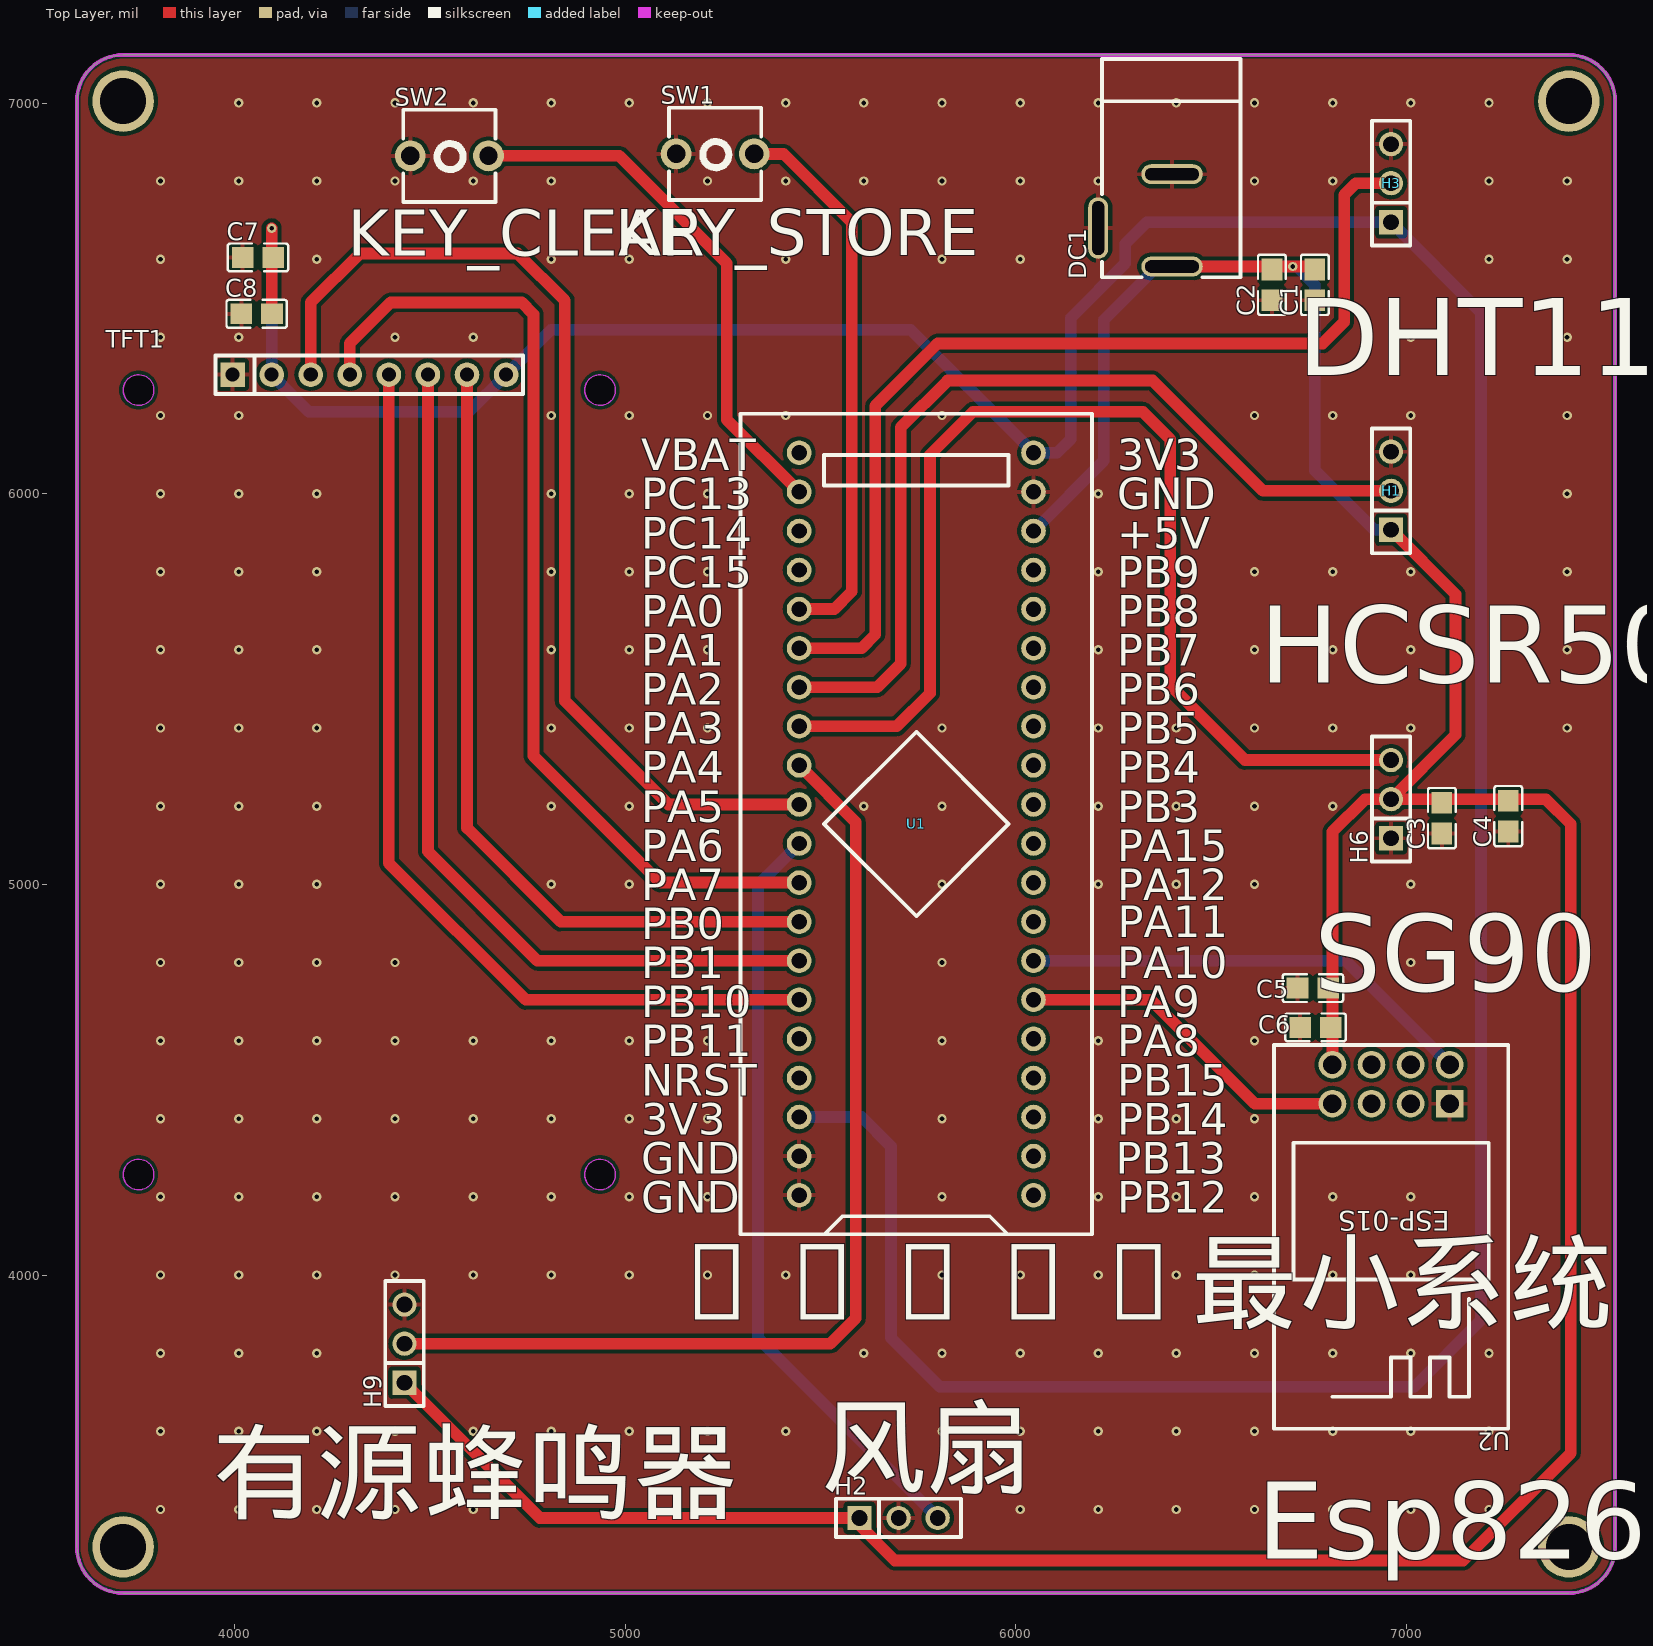
[diagram p0: Top Layer view]
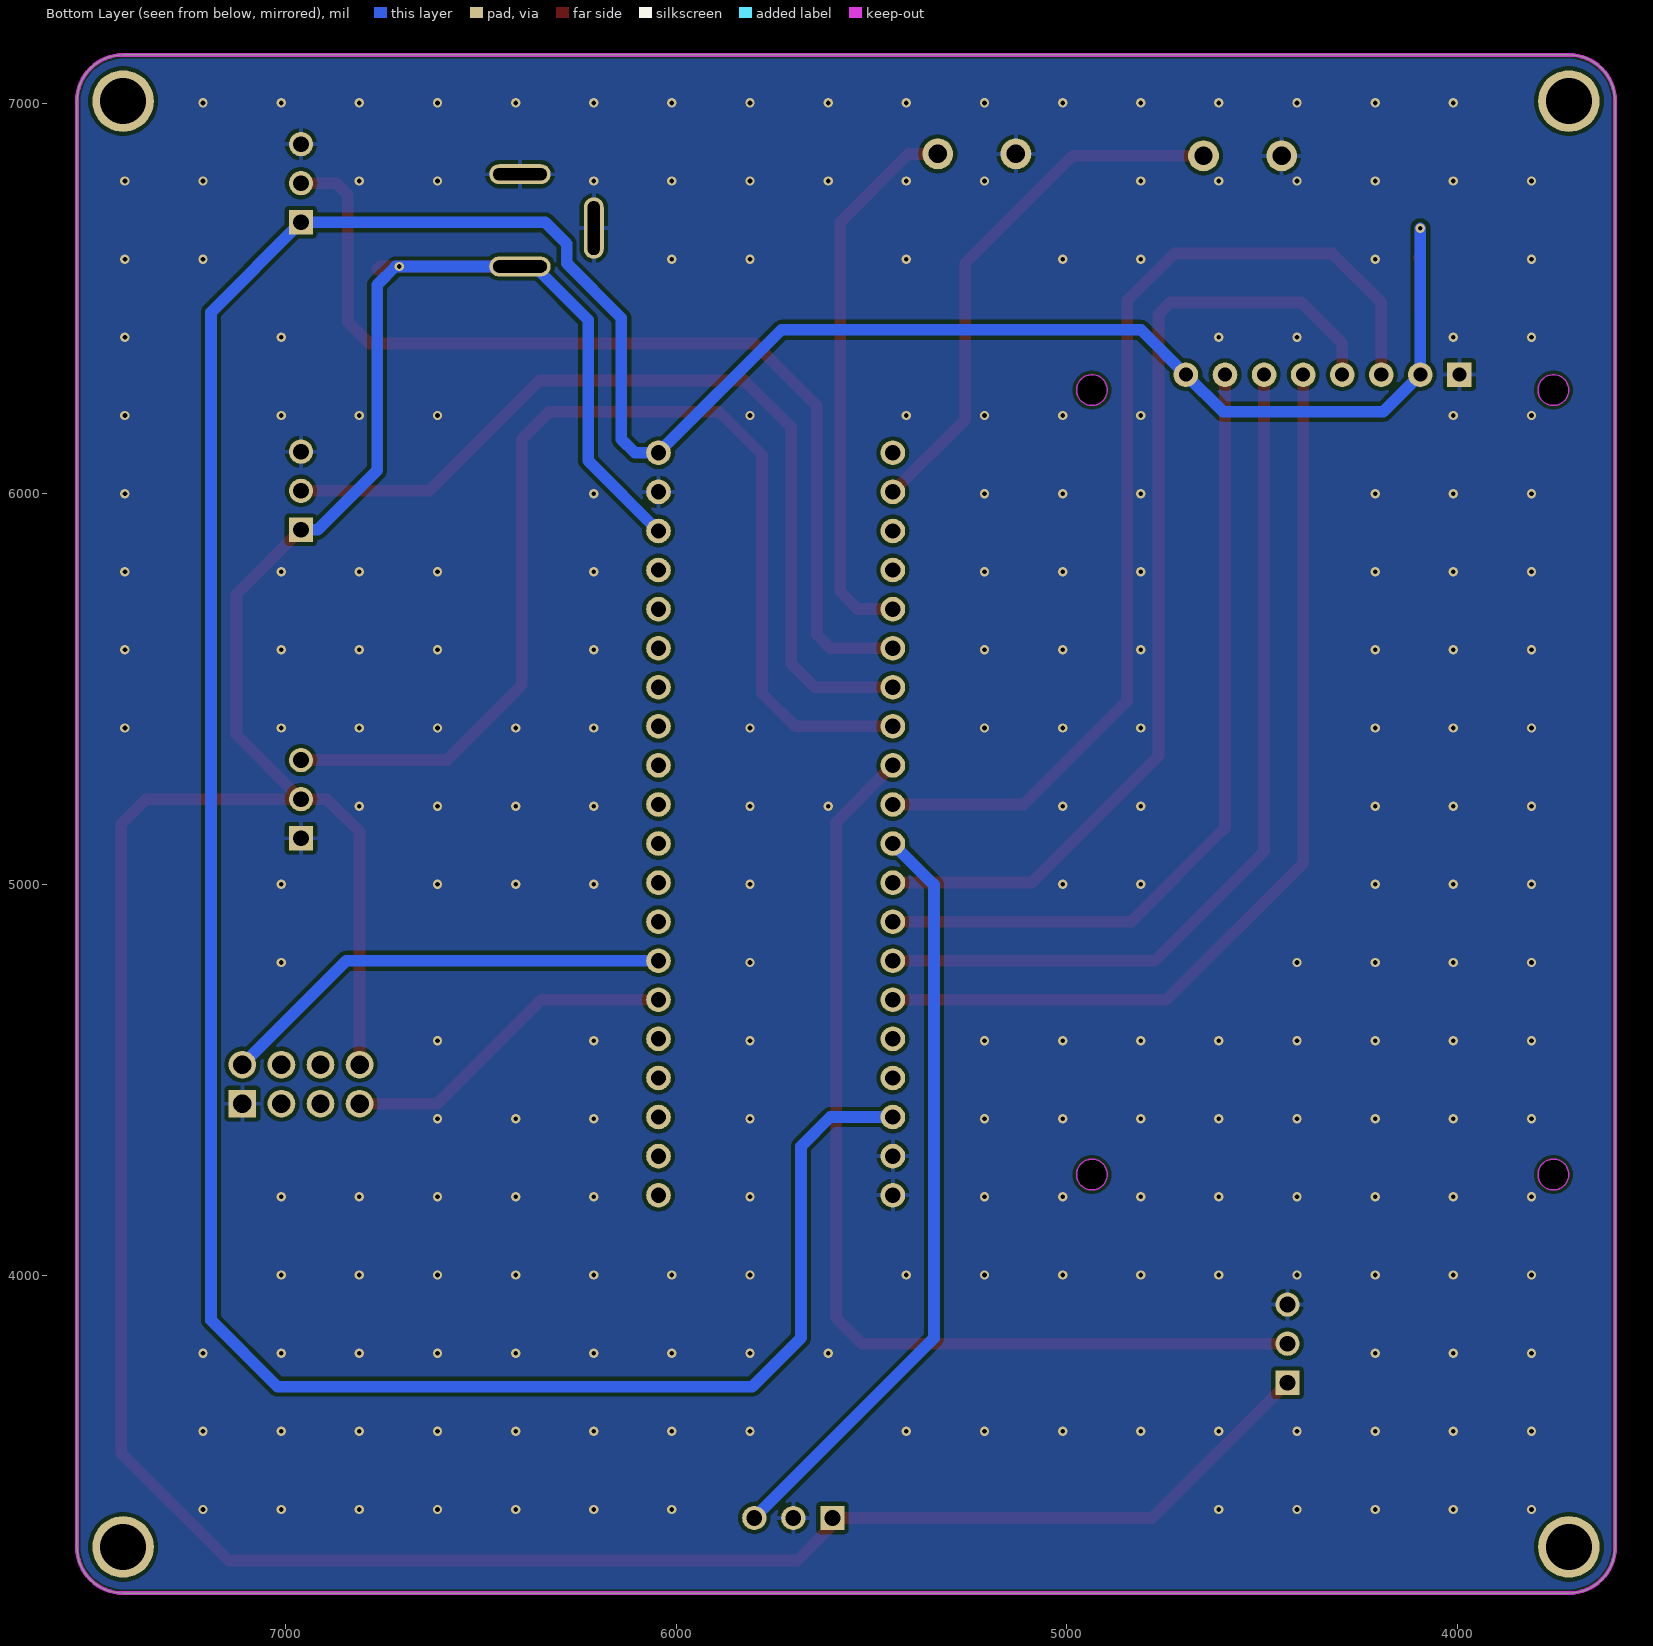
[diagram p1: Bottom Layer view, seen from below]
# Altium PCB MISC52046.pcbdoc
Units mil, origin at the board's own origin, x right, y up, seen from the top; angles counter-clockwise.
Board outline 3937.01 x 3937.01 mil, 2 copper layers (Top Layer, Bottom Layer), stack 62.206 mil thick; 19 components, 37 nets, 98 pads, 225 vias.

## Layer stack, top to bottom
Top Solder Mask Layer: solder mask 0.394, Dk 3.3
Top Layer: signal copper 1.379
Dielectric1: surface 59.449, FR4, Dk 4.5
Bottom Layer: signal copper 1.378
Bottom Solder Mask Layer: solder mask 0.394, Dk 3.3

## Board outline
3714.61,7123.5 ccw(c3714.61,7005.39) 3596.5,7005.39 3596.5,3304.61 ccw(c3714.61,3304.61) 3714.61,3186.5 7415.39,3186.5 ccw(c7415.39,3304.61) 7533.5,3304.61 7533.5,7005.39 ccw(c7415.39,7005.39) 7415.39,7123.5 3714.61,7123.5

## Design rules (kind name [scope] priority, off if disabled: settings)
BoardOutlineClearance copperThickness2oz_1 [All] p2 off: genericclearance=7.99 ignorepadtopadclearanceinfootprint=FALSE except(0: Arc-SplitContinuation Track-SplitContinuation SMDPad-SplitContinuation THPad-SplitContinuation Via-SplitContinuation Fill-SplitContinuation Region-SplitContinuation Poly-SplitContinuation Text-SplitContinuation Hole-SplitContinuation; 5.98: Arc-CutoutEdge Track-CutoutEdge SMDPad-CutoutEdge THPad-CutoutEdge Via-CutoutEdge Text-CutoutEdge; 6.9: Hole-OutlineEdge Hole-CutoutEdge; 10: Poly-OutlineEdge Poly-CutoutEdge; 11.81: Arc-OutlineEdge Track-OutlineEdge SMDPad-OutlineEdge THPad-OutlineEdge Via-OutlineEdge Fill-OutlineEdge Region-OutlineEdge Text-OutlineEdge Fill-CutoutEdge Region-CutoutEdge)
BoardOutlineClearance Plane_innerPlane_1 [All] p4 off: genericclearance=4.02 ignorepadtopadclearanceinfootprint=FALSE except(0: Arc-SplitContinuation Track-SplitContinuation SMDPad-SplitContinuation THPad-SplitContinuation Via-SplitContinuation Fill-SplitContinuation Region-SplitContinuation Poly-SplitContinuation Text-SplitContinuation Hole-SplitContinuation; 5.98: Arc-CutoutEdge Track-CutoutEdge SMDPad-CutoutEdge THPad-CutoutEdge Via-CutoutEdge Text-CutoutEdge; 6.9: Hole-OutlineEdge Hole-CutoutEdge; 10: Poly-OutlineEdge Poly-CutoutEdge; 11.81: Arc-OutlineEdge Track-OutlineEdge SMDPad-OutlineEdge THPad-OutlineEdge Via-OutlineEdge Fill-OutlineEdge Region-OutlineEdge Text-OutlineEdge Fill-CutoutEdge Region-CutoutEdge)
BoardOutlineClearance Copper_copperRegion_1 [All] p6 off: genericclearance=4.02 ignorepadtopadclearanceinfootprint=FALSE except(0: Arc-SplitContinuation Track-SplitContinuation SMDPad-SplitContinuation THPad-SplitContinuation Via-SplitContinuation Fill-SplitContinuation Region-SplitContinuation Poly-SplitContinuation Text-SplitContinuation Hole-SplitContinuation; 5.98: Arc-CutoutEdge Track-CutoutEdge SMDPad-CutoutEdge THPad-CutoutEdge Via-CutoutEdge Text-CutoutEdge; 6.9: Hole-OutlineEdge Hole-CutoutEdge; 10: Poly-OutlineEdge Poly-CutoutEdge; 11.81: Arc-OutlineEdge Track-OutlineEdge SMDPad-OutlineEdge THPad-OutlineEdge Via-OutlineEdge Fill-OutlineEdge Region-OutlineEdge Text-OutlineEdge Fill-CutoutEdge Region-CutoutEdge)
BoardOutlineClearance Copper_copperRegion_copperThickness1oz_1 [All] p8 off: genericclearance=4.02 ignorepadtopadclearanceinfootprint=FALSE except(0: Arc-SplitContinuation Track-SplitContinuation SMDPad-SplitContinuation THPad-SplitContinuation Via-SplitContinuation Fill-SplitContinuation Region-SplitContinuation Poly-SplitContinuation Text-SplitContinuation Hole-SplitContinuation; 5.98: Arc-CutoutEdge Track-CutoutEdge SMDPad-CutoutEdge THPad-CutoutEdge Via-CutoutEdge Text-CutoutEdge; 6.9: Hole-OutlineEdge Hole-CutoutEdge; 10: Poly-OutlineEdge Poly-CutoutEdge; 11.81: Arc-OutlineEdge Track-OutlineEdge SMDPad-OutlineEdge THPad-OutlineEdge Via-OutlineEdge Fill-OutlineEdge Region-OutlineEdge Text-OutlineEdge Fill-CutoutEdge Region-CutoutEdge)
BoardOutlineClearance Copper_copperRegion_Copper_copperRegion_1 [All] p10 off: genericclearance=4.02 ignorepadtopadclearanceinfootprint=FALSE except(0: Arc-SplitContinuation Track-SplitContinuation SMDPad-SplitContinuation THPad-SplitContinuation Via-SplitContinuation Fill-SplitContinuation Region-SplitContinuation Poly-SplitContinuation Text-SplitContinuation Hole-SplitContinuation; 5.98: Arc-CutoutEdge Track-CutoutEdge SMDPad-CutoutEdge THPad-CutoutEdge Via-CutoutEdge Text-CutoutEdge; 6.9: Hole-OutlineEdge Hole-CutoutEdge; 10: Poly-OutlineEdge Poly-CutoutEdge; 11.81: Arc-OutlineEdge Track-OutlineEdge SMDPad-OutlineEdge THPad-OutlineEdge Via-OutlineEdge Fill-OutlineEdge Region-OutlineEdge Text-OutlineEdge Fill-CutoutEdge Region-CutoutEdge)
BoardOutlineClearance copperThickness1oz_1 [All] p12: genericclearance=4.02 ignorepadtopadclearanceinfootprint=FALSE except(0: Arc-SplitContinuation Track-SplitContinuation SMDPad-SplitContinuation THPad-SplitContinuation Via-SplitContinuation Fill-SplitContinuation Region-SplitContinuation Poly-SplitContinuation Text-SplitContinuation Hole-SplitContinuation; 5.98: Arc-CutoutEdge Track-CutoutEdge SMDPad-CutoutEdge THPad-CutoutEdge Via-CutoutEdge Text-CutoutEdge; 6.9: Hole-OutlineEdge Hole-CutoutEdge; 10: Poly-OutlineEdge Poly-CutoutEdge; 11.81: Arc-OutlineEdge Track-OutlineEdge SMDPad-OutlineEdge THPad-OutlineEdge Via-OutlineEdge Fill-OutlineEdge Region-OutlineEdge Text-OutlineEdge Fill-CutoutEdge Region-CutoutEdge)
Clearance copperThickness2oz [All] p1 off: gap=7.99 ignorepadtopadclearanceinfootprint=FALSE except(5.98: SMDPad-Track SMDPad-SMDPad THPad-Track SMDPad-THPad THPad-THPad Track-Via SMDPad-Via THPad-Via Via-Via Fill-SMDPad Region-SMDPad Fill-THPad Region-THPad Fill-Via Region-Via Fill-Fill Fill-Region Region-Region Arc-Track Arc-SMDPad Arc-THPad Arc-Via Fill-Arc Region-Arc Arc-Arc Text-Track SMDPad-Text Text-THPad Text-Via Fill-Text Region-Text Arc-Text Text-Text; 6.9: Hole-Track Hole-SMDPad Hole-THPad Hole-Via Fill-Hole Region-Hole Hole-Arc Hole-Text; 10: Poly-Track Poly-SMDPad Poly-THPad Poly-Via Poly-Fill Poly-Region Poly-Poly Poly-Arc Poly-Text Poly-Hole; 11.81: Fill-Track Region-Track)
Clearance Plane_innerPlane [All] p3 off: gap=4.02 ignorepadtopadclearanceinfootprint=FALSE except(5.98: SMDPad-Track SMDPad-SMDPad THPad-Track SMDPad-THPad THPad-THPad Track-Via SMDPad-Via THPad-Via Via-Via Fill-SMDPad Region-SMDPad Fill-THPad Region-THPad Fill-Via Region-Via Fill-Fill Fill-Region Region-Region Arc-Track Arc-SMDPad Arc-THPad Arc-Via Fill-Arc Region-Arc Arc-Arc Text-Track SMDPad-Text Text-THPad Text-Via Fill-Text Region-Text Arc-Text Text-Text; 6.9: Hole-Track Hole-SMDPad Hole-THPad Hole-Via Fill-Hole Region-Hole Hole-Arc Hole-Text; 10: Poly-Track Poly-SMDPad Poly-THPad Poly-Via Poly-Fill Poly-Region Poly-Poly Poly-Arc Poly-Text Poly-Hole; 11.81: Fill-Track Region-Track)
Clearance Copper_copperRegion [All] p5 off: gap=4.02 ignorepadtopadclearanceinfootprint=FALSE except(5.98: SMDPad-Track SMDPad-SMDPad THPad-Track SMDPad-THPad THPad-THPad Track-Via SMDPad-Via THPad-Via Via-Via Fill-SMDPad Region-SMDPad Fill-THPad Region-THPad Fill-Via Region-Via Fill-Fill Fill-Region Region-Region Arc-Track Arc-SMDPad Arc-THPad Arc-Via Fill-Arc Region-Arc Arc-Arc Text-Track SMDPad-Text Text-THPad Text-Via Fill-Text Region-Text Arc-Text Text-Text; 6.9: Hole-Track Hole-SMDPad Hole-THPad Hole-Via Fill-Hole Region-Hole Hole-Arc Hole-Text; 10: Poly-Track Poly-SMDPad Poly-THPad Poly-Via Poly-Fill Poly-Region Poly-Poly Poly-Arc Poly-Text Poly-Hole; 11.81: Fill-Track Region-Track)
Clearance Copper_copperRegion_copperThickness1oz [All] p7 off: gap=4.02 ignorepadtopadclearanceinfootprint=FALSE except(5.98: SMDPad-Track SMDPad-SMDPad THPad-Track SMDPad-THPad THPad-THPad Track-Via SMDPad-Via THPad-Via Via-Via Fill-SMDPad Region-SMDPad Fill-THPad Region-THPad Fill-Via Region-Via Fill-Fill Fill-Region Region-Region Arc-Track Arc-SMDPad Arc-THPad Arc-Via Fill-Arc Region-Arc Arc-Arc Text-Track SMDPad-Text Text-THPad Text-Via Fill-Text Region-Text Arc-Text Text-Text; 6.9: Hole-Track Hole-SMDPad Hole-THPad Hole-Via Fill-Hole Region-Hole Hole-Arc Hole-Text; 10: Poly-Track Poly-SMDPad Poly-THPad Poly-Via Poly-Fill Poly-Region Poly-Poly Poly-Arc Poly-Text Poly-Hole; 11.81: Fill-Track Region-Track)
Clearance Copper_copperRegion_Copper_copperRegion [All] p9 off: gap=4.02 ignorepadtopadclearanceinfootprint=FALSE except(5.98: SMDPad-Track SMDPad-SMDPad THPad-Track SMDPad-THPad THPad-THPad Track-Via SMDPad-Via THPad-Via Via-Via Fill-SMDPad Region-SMDPad Fill-THPad Region-THPad Fill-Via Region-Via Fill-Fill Fill-Region Region-Region Arc-Track Arc-SMDPad Arc-THPad Arc-Via Fill-Arc Region-Arc Arc-Arc Text-Track SMDPad-Text Text-THPad Text-Via Fill-Text Region-Text Arc-Text Text-Text; 6.9: Hole-Track Hole-SMDPad Hole-THPad Hole-Via Fill-Hole Region-Hole Hole-Arc Hole-Text; 10: Poly-Track Poly-SMDPad Poly-THPad Poly-Via Poly-Fill Poly-Region Poly-Poly Poly-Arc Poly-Text Poly-Hole; 11.81: Fill-Track Region-Track)
Clearance copperThickness1oz [All] p11: gap=4.02 ignorepadtopadclearanceinfootprint=FALSE except(5.98: SMDPad-Track SMDPad-SMDPad THPad-Track SMDPad-THPad THPad-THPad Track-Via SMDPad-Via THPad-Via Via-Via Fill-SMDPad Region-SMDPad Fill-THPad Region-THPad Fill-Via Region-Via Fill-Fill Fill-Region Region-Region Arc-Track Arc-SMDPad Arc-THPad Arc-Via Fill-Arc Region-Arc Arc-Arc Text-Track SMDPad-Text Text-THPad Text-Via Fill-Text Region-Text Arc-Text Text-Text; 6.9: Hole-Track Hole-SMDPad Hole-THPad Hole-Via Fill-Hole Region-Hole Hole-Arc Hole-Text; 10: Poly-Track Poly-SMDPad Poly-THPad Poly-Via Poly-Fill Poly-Region Poly-Poly Poly-Arc Poly-Text Poly-Hole; 11.81: Fill-Track Region-Track)
DiffPairsRouting differentialPair [All] p1: maxlimit=6 minlimit=6 mostfreqgap=6 toplayer_minwidth=5 toplayer_prefwidth=10 toplayer_maxwidth=100 toplayer_mingap=6 toplayer_prefgap=6 toplayer_maxgap=6 bottomlayer_minwidth=5 bottomlayer_prefwidth=10 bottomlayer_maxwidth=100 bottomlayer_mingap=6 bottomlayer_prefgap=6 bottomlayer_maxgap=6 maxuncoupledlength=10
HoleToHoleClearance otherClearance [All] p1: gap=11.81 allowstackedmicrovias=TRUE
Length netLength [All] p1: minlimit=0 maxlimit=0
PasteMaskExpansion pasteMaskExpansion [All] p1: expansion=0
PlaneConnect innerPlane [All] p1: planeconnectstyle=Relief reliefexpansion=20 reliefentries=4 reliefconductorwidth=10 reliefairgap=10
PolygonConnect copperRegion_copperThickness1oz [All] p1 off: connectstyle=Relief reliefconductorwidth=10 reliefentries=4 polygonreliefangle="90 Angle" airgapwidth=10 via.connectstyle=Relief via.reliefconductorwidth=10 via.reliefentries=4 via.polygonreliefangle="90 Angle" via.airgapwidth=10
PolygonConnect copperRegion_Copper_copperRegion [All] p2 off: connectstyle=Relief reliefconductorwidth=10 reliefentries=4 polygonreliefangle="90 Angle" airgapwidth=10 via.connectstyle=Relief via.reliefconductorwidth=10 via.reliefentries=4 via.polygonreliefangle="90 Angle" via.airgapwidth=10
PolygonConnect copperRegion [All] p3: connectstyle=Relief reliefconductorwidth=10 reliefentries=4 polygonreliefangle="90 Angle" airgapwidth=10 via.connectstyle=Relief via.reliefconductorwidth=10 via.reliefentries=4 via.polygonreliefangle="90 Angle" via.airgapwidth=10
RoutingVias viaSize [All] p1: holewidth=12.01 width=24.02 viastyle="Through Hole" minholewidth=11.81 minwidth=19.68 maxholewidth=248.03 maxwidth=393.7
SolderMaskExpansion solderMaskExpansion [IsVia] p1: expansion=-1000 istentingtop=TRUE
SolderMaskExpansion solderMaskExpansion [All] p2: expansion=2 istentingtop=FALSE
Width copperThickness2oz_2 [All] p1 off: maxlimit=100 minlimit=8 preferedwidth=10
Width copperThickness1oz_2 [All] p2: maxlimit=100 minlimit=5 preferedwidth=10

## Components (designator, comment, footprint, x,y, rotation, side; value= is the part's Value field where it differs from the comment)
C1 "100uF" C0805 6765,6535 r90 top
C2 "100nF" C0805 6655,6535 r90 top
C3 "470uF" C0805 7090,5170 r90 top
C4 "100nF" C0805 7260,5175 r90 top
C5 "100uF" C0805 6760,4735 r0 top
C6 "100nF" C0805 6766.7,4634.47 r0 top
C7 "10uF" C0805 4060,6605 r0 top
C8 "100nF" C0805 4056.7,6460.8 r0 top
DC1 "" DC-2.0 6410,6705 r90 top
H1 "" HDR-TH_3P-P2.54-V-F 6960,6007.85 r90 top
H2 "" HDR-TH_3P-P2.54-V-F 5699.74,3378.84 r0 top
H3 "" HDR-TH_3P-P2.54-V-F 6960,6795 r90 top
H6 "" HDR-TH_3P-P2.54-V-F 6960,5218.61 r90 top
H9 "" HDR-TH_3P-P2.54-V-F 4435,3825 r90 top
SW1 "OMRON_B3F-6000" KEY-TH_2P-L6.0-W6.0-P5.00 5230,6870 r0 top
SW2 "OMRON_B3F-6000" KEY-TH_2P-L6.0-W6.0-P5.00 4550,6865 r0 top
TFT1 "1.8 TFT 128*RGB*160" LCD-TH_8P-P2.54-L56.0-W34.0_1.8-TFT 4345,6305 r0 top
U1 "STM32F103C8T6-Card" CONN-TH_L53.3-W22.9_STM32F103C8T6-CARD 5745,5155 r90 top
U2 "ESP-01S" WIFIM-TH_ESP-01S 6960,4489.11 r180 top

## Footprints (in the part's own frame and the unit in brackets; to place one, negate y for a bottom-side part, rotate by r counter-clockwise, add the part's x,y. Pads: shape width x height; smd on the part's side, far side on the other; paste and mask are expansions set on the pad)
C0805 [mm]
  rect 1.41x1.35 smd paste-100 mask+0.051: 1(-1,0) 2(1,0)
  silkscreen extent -1.96,-0.9 1.96,0.9
CONN-TH_L53.3-W22.9_STM32F103C8T6-CARD [mm]
  round 1.6 hole 1: 1(-24.13,-7.62) 2(-21.59,-7.62) 3(-19.05,-7.62) 4(-16.51,-7.62) 5(-13.97,-7.62) 6(-11.43,-7.62) 7(-8.89,-7.62) 8(-6.35,-7.62) 9(-3.81,-7.62) 10(-1.27,-7.62) 11(1.27,-7.62) 12(3.81,-7.62) 13(6.35,-7.62) 14(8.89,-7.62) 15(11.43,-7.62) 16(13.97,-7.62) 17(16.51,-7.62) 18(19.05,-7.62) 19(21.59,-7.62) 20(24.13,-7.62) 21(24.13,7.62) 22(21.59,7.62) 23(19.05,7.62) 24(16.51,7.62) 25(13.97,7.62) 26(11.43,7.62) 27(8.89,7.62) 28(6.35,7.62) 29(3.81,7.62) 30(1.27,7.62) 31(-1.27,7.62) 32(-3.81,7.62) 33(-6.35,7.62) 34(-8.89,7.62) 35(-11.43,7.62) 36(-13.97,7.62) 37(-16.51,7.62) 38(-19.05,7.62) 39(-21.59,7.62) 40(-24.13,7.62)
  silkscreen extent -26.67,-11.43 26.67,11.43
DC-2.0 [mil]
  oval 157.5x51.2 hole 31.5 slot 137.8 at 0 deg paste+0 mask+2: 2(-24.7,199.5)
  oval 51.2x157.5 hole 31.5 slot 137.8 at 90 deg paste+0 mask+2: 3(113.1,10.5) 4(-123.1,10.5)
  silkscreen extent -151,-165 408,190
HDR-TH_3P-P2.54-V-F [mil]
  rect 62x62 hole 40.16: 1(-100,0)
  round 62 hole 40.16: 2(0,0) 3(100,0)
  silkscreen extent -160,-49 160,49
KEY-TH_2P-L6.0-W6.0-P5.00 [mm]
  round 2 hole 1.2: 1(-2.54,0) 2(2.54,0)
  silkscreen extent -3,-3 3,3
LCD-TH_8P-P2.54-L56.0-W34.0_1.8-TFT [mm]
  rect 1.6x1.6 hole 0.914: 1(-8.89,0)
  round 1.6 hole 0.914: 2(-6.35,0) 3(-3.81,0) 4(-1.27,0) 5(1.27,0) 6(3.81,0) 7(6.35,0) 8(8.89,0)
  Board Outline Layer circle w0.003: c15,-1 r1
  Board Outline Layer circle w0.003: c-15,-1 r1
  Board Outline Layer circle w0.003: c15,-52 r1
  Board Outline Layer circle w0.003: c-15,-52 r1
  Board Outline Layer region: 16,-1 15.901,-1.434 15.623,-1.782 15.222,-1.975 14.777,-1.975 14.376,-1.782 14.099,-1.434 14,-1 14,-1 14.099,-0.566 14.376,-0.218 14.777,-0.025 15.222,-0.025 15.623,-0.218 15.901,-0.566 16,-1
  Board Outline Layer region: 16,-1 15.991,-1.136 15.963,-1.27 15.917,-1.398 15.854,-1.52 15.776,-1.631 15.683,-1.731 15.577,-1.817 15.46,-1.888 15.335,-1.942 15.203,-1.979 15.068,-1.998 14.932,-1.998 14.797,-1.979 14.665,-1.942 14.54,-1.888 14.423,-1.817 14.317,-1.731 14.224,-1.631 14.146,-1.52 14.083,-1.398 14.037,-1.27 14.009,-1.136 14,-1 14.009,-0.864 14.037,-0.73 14.083,-0.602 14.146,-0.48 14.224,-0.369 14.317,-0.269 14.423,-0.183 14.54,-0.112 14.665,-0.058 14.797,-0.021 14.932,-0.002 15.068,-0.002 15.203,-0.021 15.335,-0.058 15.46,-0.112 15.577,-0.183 15.683,-0.269 15.776,-0.369 15.854,-0.48 15.917,-0.602 15.963,-0.73 15.991,-0.864
  Board Outline Layer region: -14,-1 -14.099,-1.434 -14.376,-1.782 -14.777,-1.975 -15.222,-1.975 -15.623,-1.782 -15.901,-1.434 -16,-1 -16,-1 -15.901,-0.566 -15.623,-0.218 -15.222,-0.025 -14.777,-0.025 -14.376,-0.218 -14.099,-0.566 -14,-1
  Board Outline Layer region: -14,-1 -14.009,-1.136 -14.037,-1.27 -14.083,-1.398 -14.146,-1.52 -14.224,-1.631 -14.317,-1.731 -14.423,-1.817 -14.54,-1.888 -14.665,-1.942 -14.797,-1.979 -14.932,-1.998 -15.068,-1.998 -15.203,-1.979 -15.335,-1.942 -15.46,-1.888 -15.577,-1.817 -15.683,-1.731 -15.776,-1.631 -15.854,-1.52 -15.917,-1.398 -15.963,-1.27 -15.991,-1.136 -16,-1 -15.991,-0.864 -15.963,-0.73 -15.917,-0.602 -15.854,-0.48 -15.776,-0.369 -15.683,-0.269 -15.577,-0.183 -15.46,-0.112 -15.335,-0.058 -15.203,-0.021 -15.068,-0.002 -14.932,-0.002 -14.797,-0.021 -14.665,-0.058 -14.54,-0.112 -14.423,-0.183 -14.317,-0.269 -14.224,-0.369 -14.146,-0.48 -14.083,-0.602 -14.037,-0.73 -14.009,-0.864
  Board Outline Layer region: 16,-52 15.901,-52.434 15.623,-52.782 15.222,-52.975 14.777,-52.975 14.376,-52.782 14.099,-52.434 14,-52 14,-52 14.099,-51.566 14.376,-51.218 14.777,-51.025 15.222,-51.025 15.623,-51.218 15.901,-51.566 16,-52
  Board Outline Layer region: 16,-52 15.991,-52.136 15.963,-52.27 15.917,-52.398 15.854,-52.519 15.776,-52.631 15.683,-52.731 15.577,-52.817 15.46,-52.888 15.335,-52.942 15.203,-52.979 15.068,-52.998 14.932,-52.998 14.797,-52.979 14.665,-52.942 14.54,-52.888 14.423,-52.817 14.317,-52.731 14.224,-52.631 14.146,-52.519 14.083,-52.398 14.037,-52.27 14.009,-52.136 14,-52 14.009,-51.864 14.037,-51.73 14.083,-51.601 14.146,-51.48 14.224,-51.369 14.317,-51.269 14.423,-51.183 14.54,-51.112 14.665,-51.058 14.797,-51.021 14.932,-51.002 15.068,-51.002 15.203,-51.021 15.335,-51.058 15.46,-51.112 15.577,-51.183 15.683,-51.269 15.776,-51.369 15.854,-51.48 15.917,-51.601 15.963,-51.73 15.991,-51.864
  Board Outline Layer region: -14,-52 -14.099,-52.434 -14.376,-52.782 -14.777,-52.975 -15.222,-52.975 -15.623,-52.782 -15.901,-52.434 -16,-52 -16,-52 -15.901,-51.566 -15.623,-51.218 -15.222,-51.025 -14.777,-51.025 -14.376,-51.218 -14.099,-51.566 -14,-52
  Board Outline Layer region: -14,-52 -14.009,-52.136 -14.037,-52.27 -14.083,-52.398 -14.146,-52.519 -14.224,-52.631 -14.317,-52.731 -14.423,-52.817 -14.54,-52.888 -14.665,-52.942 -14.797,-52.979 -14.932,-52.998 -15.068,-52.998 -15.203,-52.979 -15.335,-52.942 -15.46,-52.888 -15.577,-52.817 -15.683,-52.731 -15.776,-52.631 -15.854,-52.519 -15.917,-52.398 -15.963,-52.27 -15.991,-52.136 -16,-52 -15.991,-51.864 -15.963,-51.73 -15.917,-51.601 -15.854,-51.48 -15.776,-51.369 -15.683,-51.269 -15.577,-51.183 -15.46,-51.112 -15.335,-51.058 -15.203,-51.021 -15.068,-51.002 -14.932,-51.002 -14.797,-51.021 -14.665,-51.058 -14.54,-51.112 -14.423,-51.183 -14.317,-51.269 -14.224,-51.369 -14.146,-51.48 -14.083,-51.601 -14.037,-51.73 -14.009,-51.864
  Multi-Layer board cut-out: 16,-1 15.901,-1.434 15.623,-1.782 15.222,-1.975 14.777,-1.975 14.376,-1.782 14.099,-1.434 14,-1 14,-1 14.099,-0.566 14.376,-0.218 14.777,-0.025 15.222,-0.025 15.623,-0.218 15.901,-0.566 16,-1
  Multi-Layer board cut-out: -14,-1 -14.099,-1.434 -14.376,-1.782 -14.777,-1.975 -15.222,-1.975 -15.623,-1.782 -15.901,-1.434 -16,-1 -16,-1 -15.901,-0.566 -15.623,-0.218 -15.222,-0.025 -14.777,-0.025 -14.376,-0.218 -14.099,-0.566 -14,-1
  Multi-Layer board cut-out: 16,-52 15.901,-52.434 15.623,-52.782 15.222,-52.975 14.777,-52.975 14.376,-52.782 14.099,-52.434 14,-52 14,-52 14.099,-51.566 14.376,-51.218 14.777,-51.025 15.222,-51.025 15.623,-51.218 15.901,-51.566 16,-52
  Multi-Layer board cut-out: -14,-52 -14.099,-52.434 -14.376,-52.782 -14.777,-52.975 -15.222,-52.975 -15.623,-52.782 -15.901,-52.434 -16,-52 -16,-52 -15.901,-51.566 -15.623,-51.218 -15.222,-51.025 -14.777,-51.025 -14.376,-51.218 -14.099,-51.566 -14,-52
  silkscreen extent -10,-1.25 10,1.25
WIFIM-TH_ESP-01S [mm]
  rect 1.8x1.8 hole 1.2: 1(-3.81,1.27)
  round 1.8 hole 1.2: 2(-1.27,1.27) 3(1.27,1.27) 4(3.81,1.27) 5(3.81,-1.27) 6(1.27,-1.27) 7(-1.27,-1.27) 8(-3.81,-1.27)
  silkscreen extent -7.62,-2.54 7.62,22.4

## Free pads (board coordinates)
  round 157.48 hole 118.11: 1(3714.61,7005.39) 1(3714.61,3304.61) 1(7415.39,7005.39) 1(7415.39,3304.61)

## Via types
v1: diameter 24.02, hole 12, Top Layer to Bottom Layer, 225 vias

## Nets (pads, with @x,y where several pads share a name; then routed paths per layer and width w, separated by ;. In a path a pad name is that pad's centre, name@x,y a point inside that pad or via, vN(x,y) a via of type N, cw(c..) or ccw(c..) an arc to the next point about the centre after c; other vN are vias at no path point)
+5V: C1.2 C2.2 C3.2 C4.2 C5.2 C6.2 DC1.4 H1.1 H2.1 H6.2 H9.1 U1.18 U2.5 | length 9333.4
  Top Layer w30: H9.1 4781.16,3378.84 H2.1 5599.74,3360.26 5690,3270 7145,3270 7420,3545 7420,5155 7356.39,5218.61 H6.2 ; DC1.4 v1(6708.68,6581.9) 6757.47,6581.9 C1.2 ; U2.5 6810,5135 6893.61,5218.61 H6.2 ; H1.1 7125,5742.85 7125,5383.61 H6.2
  Bottom Layer w30: U1.18 6225,6085 6225,6445 6361.9,6581.9 DC1.4 6718.1,6581.9 6765,6535 6765,6060 6917.15,5907.85 H1.1
GND: C1.1 C2.1 C3.1 C4.1 C5.1 C6.1 C7.1 C8.1 DC1.2 DC1.3 H1.3 H2.2 H3.3 H6.1 H9.3 SW1.1 SW2.1 TFT1.1 U1.19 U1.39 U1.40 U2.1
  other v1: 3810.6,3400.6 4010.6,3400.6 4210.6,3400.6 4410.6,3400.6 4610.6,3400.6 6010.6,3400.6 6210.6,3400.6 6410.6,3400.6 6610.6,3400.6 6810.6,3400.6 7010.6,3400.6 7210.6,3400.6 3810.6,3600.6 4010.6,3600.6 4210.6,3600.6 4410.6,3600.6 4610.6,3600.6 4810.6,3600.6 5010.6,3600.6 5210.6,3600.6 5410.6,3600.6 5810.6,3600.6 6010.6,3600.6 6210.6,3600.6 6410.6,3600.6 6610.6,3600.6 6810.6,3600.6 7010.6,3600.6 7210.6,3600.6 3810.6,3800.6 4010.6,3800.6 4210.6,3800.6 5610.6,3800.6 5810.6,3800.6 6010.6,3800.6 6210.6,3800.6 6410.6,3800.6 6610.6,3800.6 6810.6,3800.6 7010.6,3800.6 7210.6,3800.6 3810.6,4000.6 4010.6,4000.6 4210.6,4000.6 4410.6,4000.6 4610.6,4000.6 4810.6,4000.6 5010.6,4000.6 5210.6,4000.6 5410.6,4000.6 5810.6,4000.6 6010.6,4000.6 6210.6,4000.6 6410.6,4000.6 6610.6,4000.6 6810.6,4000.6 7010.6,4000.6 3810.6,4200.6 4010.6,4200.6 4210.6,4200.6 4410.6,4200.6 4610.6,4200.6 4810.6,4200.6 5010.6,4200.6 5210.6,4200.6 5810.6,4200.6 6210.6,4200.6 6410.6,4200.6 6610.6,4200.6 6810.6,4200.6 7010.6,4200.6 3810.6,4400.6 4010.6,4400.6 4210.6,4400.6 4410.6,4400.6 4610.6,4400.6 4810.6,4400.6 5010.6,4400.6 5210.6,4400.6 5810.6,4400.6 6210.6,4400.6 6410.6,4400.6 6610.6,4400.6 3810.6,4600.6 4010.6,4600.6 4210.6,4600.6 4410.6,4600.6 4610.6,4600.6 4810.6,4600.6 5010.6,4600.6 5210.6,4600.6 5810.6,4600.6 6210.6,4600.6 6610.6,4600.6 3810.6,4800.6 4010.6,4800.6 4210.6,4800.6 4410.6,4800.6 5810.6,4800.6 7010.6,4800.6 3810.6,5000.6 4010.6,5000.6 4210.6,5000.6 4810.6,5000.6 5010.6,5000.6 5810.6,5000.6 6210.6,5000.6 6410.6,5000.6 6610.6,5000.6 7010.6,5000.6 3810.6,5200.6 4010.6,5200.6 4210.6,5200.6 4810.6,5200.6 5010.6,5200.6 5610.6,5200.6 5810.6,5200.6 6210.6,5200.6 6410.6,5200.6 6610.6,5200.6 6810.6,5200.6 3810.6,5400.6 4010.6,5400.6 4210.6,5400.6 4810.6,5400.6 5010.6,5400.6 5210.6,5400.6 5810.6,5400.6 6210.6,5400.6 6410.6,5400.6 6610.6,5400.6 6810.6,5400.6 7010.6,5400.6 7410.6,5400.6 3810.6,5600.6 4010.6,5600.6 4210.6,5600.6 4810.6,5600.6 5010.6,5600.6 5210.6,5600.6 6210.6,5600.6 6610.6,5600.6 6810.6,5600.6 7010.6,5600.6 7410.6,5600.6 3810.6,5800.6 4010.6,5800.6 4210.6,5800.6 4810.6,5800.6 5010.6,5800.6 5210.6,5800.6 6210.6,5800.6 6610.6,5800.6 6810.6,5800.6 7010.6,5800.6 7410.6,5800.6 3810.6,6000.6 4010.6,6000.6 4210.6,6000.6 4810.6,6000.6 5010.6,6000.6 5210.6,6000.6 6210.6,6000.6 7410.6,6000.6 3810.6,6200.6 4010.6,6200.6 4810.6,6200.6 5010.6,6200.6 5210.6,6200.6 5410.6,6200.6 5810.6,6200.6 6610.6,6200.6 6810.6,6200.6 7010.6,6200.6 7410.6,6200.6 3810.6,6400.6 4010.6,6400.6 4410.6,6400.6 4610.6,6400.6 7010.6,6400.6 7410.6,6400.6 3810.6,6600.6 4210.6,6600.6 4810.6,6600.6 5010.6,6600.6 5410.6,6600.6 5810.6,6600.6 6010.6,6600.6 7210.6,6600.6 7410.6,6600.6 3810.6,6800.6 4010.6,6800.6 4210.6,6800.6 4410.6,6800.6 4610.6,6800.6 4810.6,6800.6 5210.6,6800.6 5410.6,6800.6 5610.6,6800.6 5810.6,6800.6 6010.6,6800.6 6210.6,6800.6 6610.6,6800.6 6810.6,6800.6 7210.6,6800.6 7410.6,6800.6 4010.6,7000.6 4210.6,7000.6 4410.6,7000.6 4610.6,7000.6 4810.6,7000.6 5010.6,7000.6 5210.6,7000.6 5410.6,7000.6 5610.6,7000.6 5810.6,7000.6 6010.6,7000.6 6210.6,7000.6 6410.6,7000.6 6610.6,7000.6 6810.6,7000.6 7010.6,7000.6 7210.6,7000.6
NRST: U1.37
PA0: SW1.2 U1.25 | length 1421.1
  Top Layer w30: SW1.2 5405,6870 5580,6695 5580,5750 5535,5705 U1.25
PA1: H3.2 U1.26 | length 2541
  Top Layer w30: U1.26 5605,5605 5640,5640 5640,6225 5800,6385 6785,6385 6840,6440 6840,6765 6870,6795 H3.2
PA2: H1.2 U1.27 | length 2311.4
  Top Layer w30: U1.27 5645,5505 5705,5565 5705,6170 5825,6290 6350,6290 6632.15,6007.85 H1.2
PA3: H6.3 U1.28 | length 2944
  Top Layer w30: U1.28 5695,5405 5780,5490 5780,6100 5890,6210 6325,6210 6395,6140 6395,5510 6586.39,5318.61 H6.3
PA4: H9.2 U1.29 | length 2657
  Top Layer w30: H9.2 5525,3825 5590,3890 5590,5160 U1.29
PA5: TFT1.3 U1.30 | length 2671.2
  Top Layer w30: TFT1.3 4195,6490 4320,6615 4725,6615 4845,6495 4845,5470 5110,5205 U1.30
PA6: H2.3 U1.31 | length 1960.1
  Bottom Layer w30: U1.31 5340,5000 5340,3838.58 H2.3
PA7: TFT1.4 U1.32 | length 2550.5
  Top Layer w30: TFT1.4 4295,6385 4400,6490 4735,6490 4765,6460 4765,5330 5090,5005 U1.32
PA8: U1.5
PA9: U1.6 U2.4 | length 875.1
  Top Layer w30: U1.6 6345,4705 6610.89,4439.11 U2.4
PA10: U1.7 U2.8 | length 1175.1
  Bottom Layer w30: U1.7 6844.11,4805 U2.8
PA11: U1.8
PA12: U1.9
PA15: U1.10
PB0: TFT1.7 U1.33 | length 2109.4
  Top Layer w30: TFT1.7 4595,5145 4835,4905 U1.33
PB1: TFT1.6 U1.34 | length 2286
  Top Layer w30: TFT1.6 4495,5085 4775,4805 U1.34
PB3: U1.11
PB4: U1.12
PB5: U1.13
PB6: U1.14
PB7: U1.15
PB8: U1.16
PB9: U1.17
PB10: TFT1.5 U1.35 | length 2445
  Top Layer w30: TFT1.5 4395,5055 4745,4705 U1.35
PB11: U1.36
PB12: U1.1
PB13: U1.2
PB14: U1.3
PB15: U1.4
PC13: SW2.2 U1.22 | length 1385.5
  Top Layer w30: SW2.2 4985,6865 5260,6590 5260,6190 U1.22
PC14: U1.23
PC15: U1.24
VBAT: U1.21
VCC: C7.2 C8.2 H3.1 TFT1.2 TFT1.8 U1.20 U1.38 | length 9471
  Top Layer w30: C8.2@4095,6460.8 C7.2@4095,6600.63 ; v1(4095,6680) C7.2@4095,6600.63 ; C7.2 C7.2@4095,6600.63
  Bottom Layer w30: v1(4095,6680) TFT1.2 4190,6210 4600,6210 TFT1.8 4810,6420 5730,6420 U1.20 6105,6105 6140,6140 6140,6450 6280,6590 6280,6640 6335,6695 H3.1 7190,6465 7190,3885 7020,3715 5805,3715 5680,3840 5680,4330 5605,4405 U1.38
pads on no net: U2.2 U2.3 U2.6 U2.7

## Polygon pours and split planes (outlines as drawn)
GND on Bottom Layer (solid, remove dead copper, pour order 2): 3525,7245 3525,3080 7700,3080 7700,7245
GND on Top Layer (solid, remove dead copper, pour order 2): 3000,7415 3000,3000 7930,3000 7930,7415

## Keep-outs
Board Outline Layer:
  the board outline again, w10

## Silkscreen, mask and mechanical layers (free items; w line width, h text height)
Top Silkscreen Layer:
  text "KEY_STORE" at 4974.25,6610.77 h118.11
  text "KEY_CLEAR" at 4290,6610 h118.11
  text "DHT11" at 6721.39,6304.04 h196.85
  text "VBAT" at 5040.95,6060 h80
  text "3V3" at 6259.16,6060 h80
  text "PC13" at 5040.95,5960 h80
  text "GND" at 6259.16,5960 h80
  text "PC14" at 5040.95,5860 h80
  text "+5V" at 6259.16,5860 h80
  text "PC15" at 5040.95,5760 h80
  text "PB9" at 6259.16,5760 h80
  text "PA0" at 5040.95,5660 h80
  text "PB8" at 6259.16,5660 h80
  text "PA1" at 5040.95,5560 h80
  text "PB7" at 6259.16,5560 h80
  text "HCSR501" at 6624.01,5516.59 h196.85
  text "PA2" at 5040.95,5460 h80
  text "PB6" at 6259.16,5460 h80
  text "PA3" at 5040.95,5360 h80
  text "PB5" at 6259.16,5360 h80
  text "PA4" at 5040.95,5260 h80
  text "PB4" at 6259.16,5260 h80
  text "PA5" at 5040.95,5160 h80
  text "PB3" at 6259.16,5160 h80
  text "PA6" at 5040.95,5060 h80
  text "PA15" at 6259.16,5060 h80
  text "PA7" at 5040.95,4960 h80
  text "PA12" at 6259.16,4960 h80
  text "PA11" at 6260.95,4865 h80
  text "PB0" at 5040.95,4860 h80
  text "PB1" at 5040.95,4760 h80
  text "PA10" at 6259.16,4760 h80
  text "SG90" at 6764.04,4727.35 h196.85
  text "PB10" at 5040.95,4660 h80
  text "PA9" at 6259.16,4660 h80
  text "PB11" at 5040.95,4560 h80
  text "PA8" at 6259.16,4560 h80
  text "NRST" at 5040.95,4460 h80
  text "PB15" at 6259.16,4460 h80
  text "3V3" at 5040.95,4360 h80
  text "PB14" at 6259.16,4360 h80
  text "GND" at 5040.95,4260 h80
  text "PB13" at 6255.95,4260 h80
  text "GND" at 5040.95,4160 h80
  text "PB12" at 6259.16,4160 h80
  text "STM32最小系统" at 5099.45,3886.57 h196.85
  text "风扇" at 5500,3465 h196.85
  text "有源蜂鸣器" at 3940,3400 h196.85
  text "Esp8266" at 6618.05,3275 h196.85